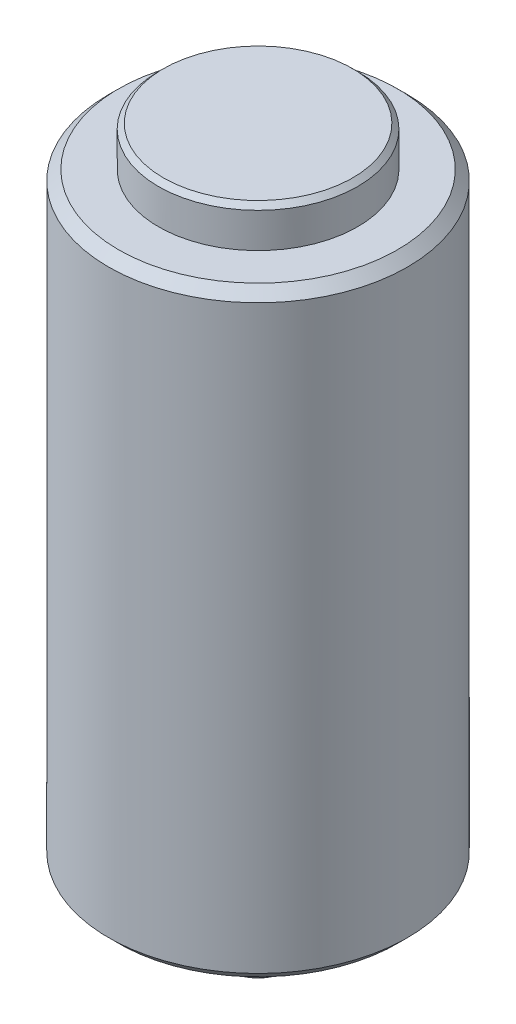
SolidWorks part; units mm, degrees
material "20#"
ref_plane "Front Plane" through (0, 0, 0) normal (0, 0, 1) x (1, 0, 0)
ref_plane "Top Plane" through (0, 0, 0) normal (0, 1, 0) x (1, 0, 0)
ref_plane "Right Plane" through (0, 0, 0) normal (1, 0, 0) x (0, 0, -1)
sketch "Sketch1" plane through (0, 0, 0) normal (0, 0, 1) x (1, 0, 0)
  line L0 (471.6666, -1187.1705) -> (471.6666, -1114.8705) construction
  line L1 (481.6666, -1187.1705) -> (381.6666, -1187.1705) construction
  line L2 (221.6666, -1114.8705) -> (535.1666, -1114.8705) construction
  line L3 (477.9166, -1175.1705) -> (477.9166, -1172.8705) construction
  line L4 (486.6666, -1172.8705) -> (486.6666, -1112.5705)
  line L5 (484.6666, -1172.8705) -> (378.6666, -1172.8705) construction
  line L6 (-561.3334, -1112.5705) -> (688.6666, -1112.5705) construction
  line L7 (486.6666, -1112.5705) -> (481.6666, -1112.5705)
  line L8 (481.6666, -1112.5705) -> (481.6666, -1108.5705)
  line L9 (481.6666, -1108.5705) -> (471.6666, -1108.5705)
  line L10 (471.6666, -1114.8705) -> (471.6666, -1108.0705) construction
  line L11 (-561.3334, -1108.0705) -> (688.6666, -1108.0705) construction
  line L12 (486.6666, -1172.8705) -> (477.9166, -1172.8705)
  line L13 (477.9166, -1172.8705) -> (477.9166, -1174.8705)
  line L14 (477.9166, -1174.8705) -> (475.9166, -1174.8705)
  line L15 (475.9166, -1174.8705) -> (475.9166, -1180.5705)
  line L16 (475.9166, -1180.5705) -> (471.6666, -1180.5705)
  line L17 (471.6666, -1180.5705) -> (471.6666, -1108.5705)
  dimension "D1" = 6.25
  dimension "D2" = 30
  dimension "D3" = 12.5
  dimension "D4" = 8.5
  dimension "D5" = 2
  dimension "D6" = 5.7
  dimension "D7" = 60.3
  dimension "D8" = 20
  dimension "D9" = 4
revolve "Revolve1" add sketch "Sketch1" angle 360 about L17
chamfer "Chamfer1" distance 1 angle 45 3 edges at (471.6666, -1180.5705, -4.25) (471.6666, -1112.5705, -15) (471.6666, -1172.8705, -15)
chamfer "Chamfer2" distance 0.5 angle 45 2 edges at (471.6666, -1108.5705, -10) (471.6666, -1174.8705, -6.25)
